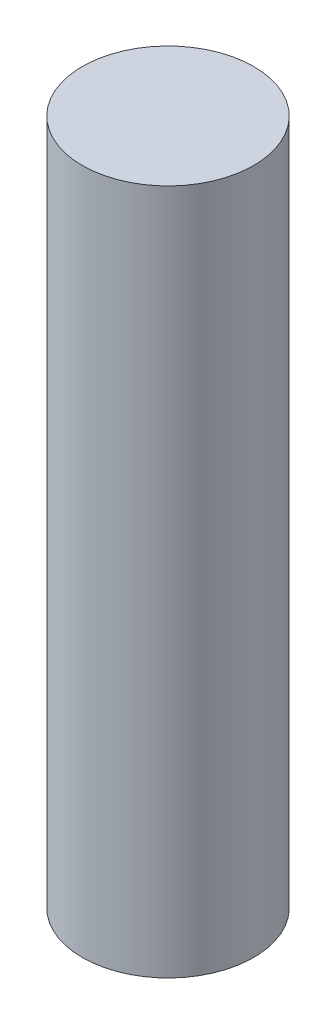
SolidWorks part; units mm, degrees
ref_plane "Front Plane" through (0, 0, 0) normal (0, 0, 1) x (1, 0, 0)
ref_plane "Top Plane" through (0, 0, 0) normal (0, 1, 0) x (1, 0, 0)
ref_plane "Right Plane" through (0, 0, 0) normal (1, 0, 0) x (0, 0, -1)
sketch "Sketch1" plane through (0, 0, 0) normal (0, 1, 0) x (1, 0, 0)
  circle A0 centre (0, 0) radius 12.5
  dimension "D1" = 25
extrude "Boss-Extrude1" add sketch "Sketch1" along normal blind 100
